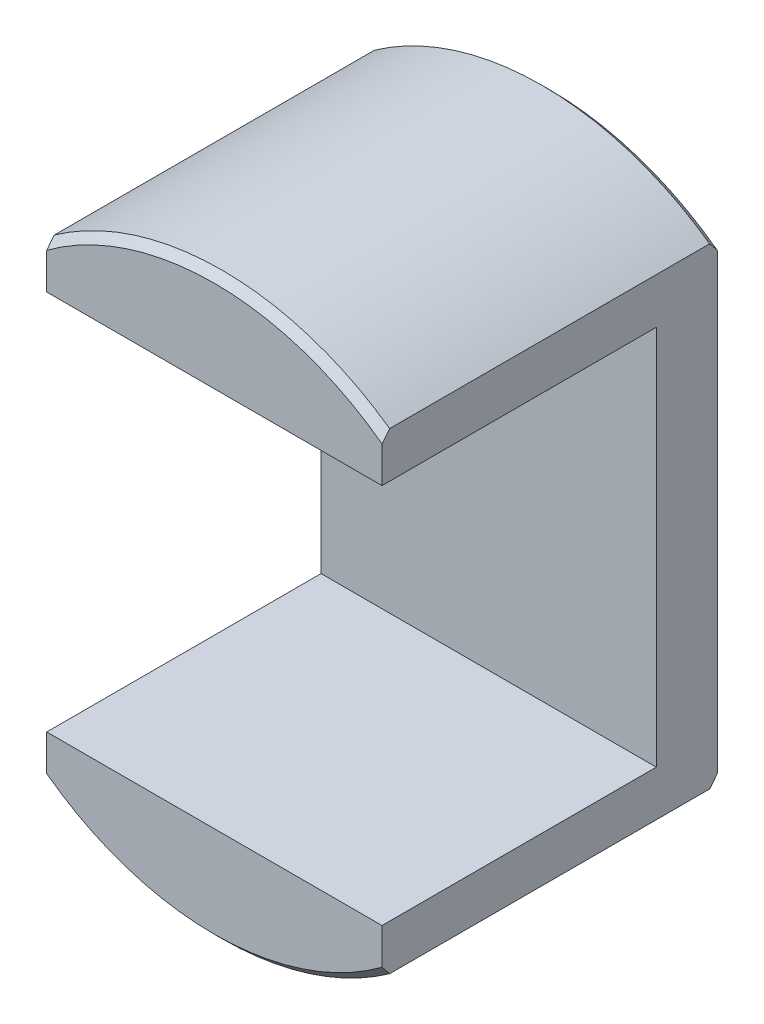
from build123d import *

# Parameters (mm, degrees)
BOSS_EXTRUDE1_DEPTH = 22
SKETCH2_W           = 22
SKETCH2_H           = 25
CUT_EXTRUDE1_DEPTH  = 18
CHAMFER1_SIZE       = 0.5


with BuildPart() as part:
    # Sketch1 → Boss-Extrude1 (new body)
    with BuildSketch(Plane.XY):
        with BuildLine():
            Line((11, -15.491933385), (11, 15.491933385))
            ThreePointArc((11, 15.491933385), (0, 19), (-11, 15.491933385))
            Line((-11, 15.491933385), (-11, -15.491933385))
            ThreePointArc((-11, -15.491933385), (0, -19), (11, -15.491933385))
        make_face()
    extrude(amount=BOSS_EXTRUDE1_DEPTH)

    # Sketch2 → Cut-Extrude1 (cut)
    with BuildSketch(Plane.XY.offset(22)):
        Rectangle(SKETCH2_W, SKETCH2_H)
    extrude(amount=-CUT_EXTRUDE1_DEPTH, mode=Mode.SUBTRACT)

    # Chamfer1
    chamfer1_edges = [part.edges().sort_by_distance(p)[0] for p in [
        (0, 19, 22),
        (0, -19, 22),
        (0, 19, 0),
        (0, -19, 0),
    ]]
    chamfer(chamfer1_edges, length=CHAMFER1_SIZE)


solid = part.part
